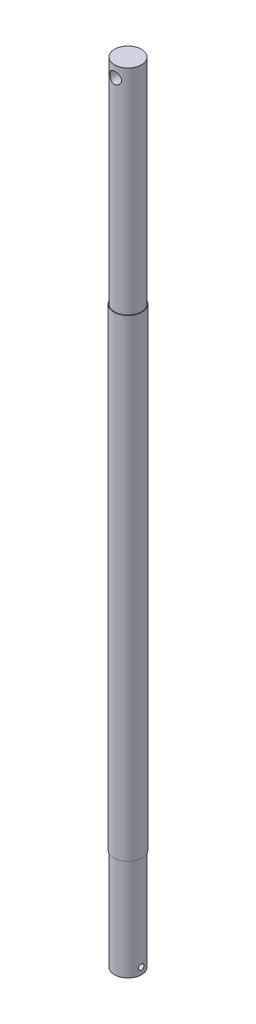
SolidWorks part; units mm, degrees
material "45#"
ref_plane "Front Plane" through (0, 0, 0) normal (0, 0, 1) x (1, 0, 0)
ref_plane "Top Plane" through (0, 0, 0) normal (0, 1, 0) x (1, 0, 0)
ref_plane "Right Plane" through (0, 0, 0) normal (1, 0, 0) x (0, 0, -1)
sketch "Sketch1" plane through (0, 0, 0) normal (0, 1, 0) x (1, 0, 0)
  circle A0 centre (0, 0) radius 12
  dimension "D1" = 24
extrude "Boss-Extrude1" add sketch "Sketch1" along normal blind 90
cosmetic thread "Cosmetic Thread1" parameters "D1"=90, "D2"=20.752
sketch "Sketch2" plane through (0, 90, 0) normal (0, 1, 0) x (1, 0, 0)
  circle A0 centre (0, 0) radius 12.5
  dimension "D1" = 25
extrude "Boss-Extrude2" add sketch "Sketch2" along normal blind 420
sketch "Sketch3" plane through (0, 510, 0) normal (0, 1, 0) x (1, 0, 0)
  circle A0 centre (0, 0) radius 12
  dimension "D1" = 24
extrude "Boss-Extrude3" add sketch "Sketch3" along normal blind 190
cosmetic thread "Cosmetic Thread2" parameters "D1"=190, "D2"=20.752
sketch "Sketch4" plane through (0, 0, 0) normal (0, 0, 1) x (1, 0, 0)
  line L0 (12, 700) -> (-12, 700) construction
  line L1 (0, 690) -> (0, 700) construction
  circle A0 centre (0, 690) radius 5.1
  dimension "D1" = 10.2
  dimension "D2" = 10
extrude "Cut-Extrude1" cut sketch "Sketch4" against normal through all both and the other way through all
sketch "Sketch5" plane through (0, 0, 0) normal (1, 0, 0) x (0, 0, -1)
  line L0 (0, 0) -> (0, 6) construction
  circle A0 centre (0, 6) radius 2.5
  dimension "D1" = 6
  dimension "D2" = 5
extrude "Cut-Extrude2" cut sketch "Sketch5" against normal through all both and the other way through all
